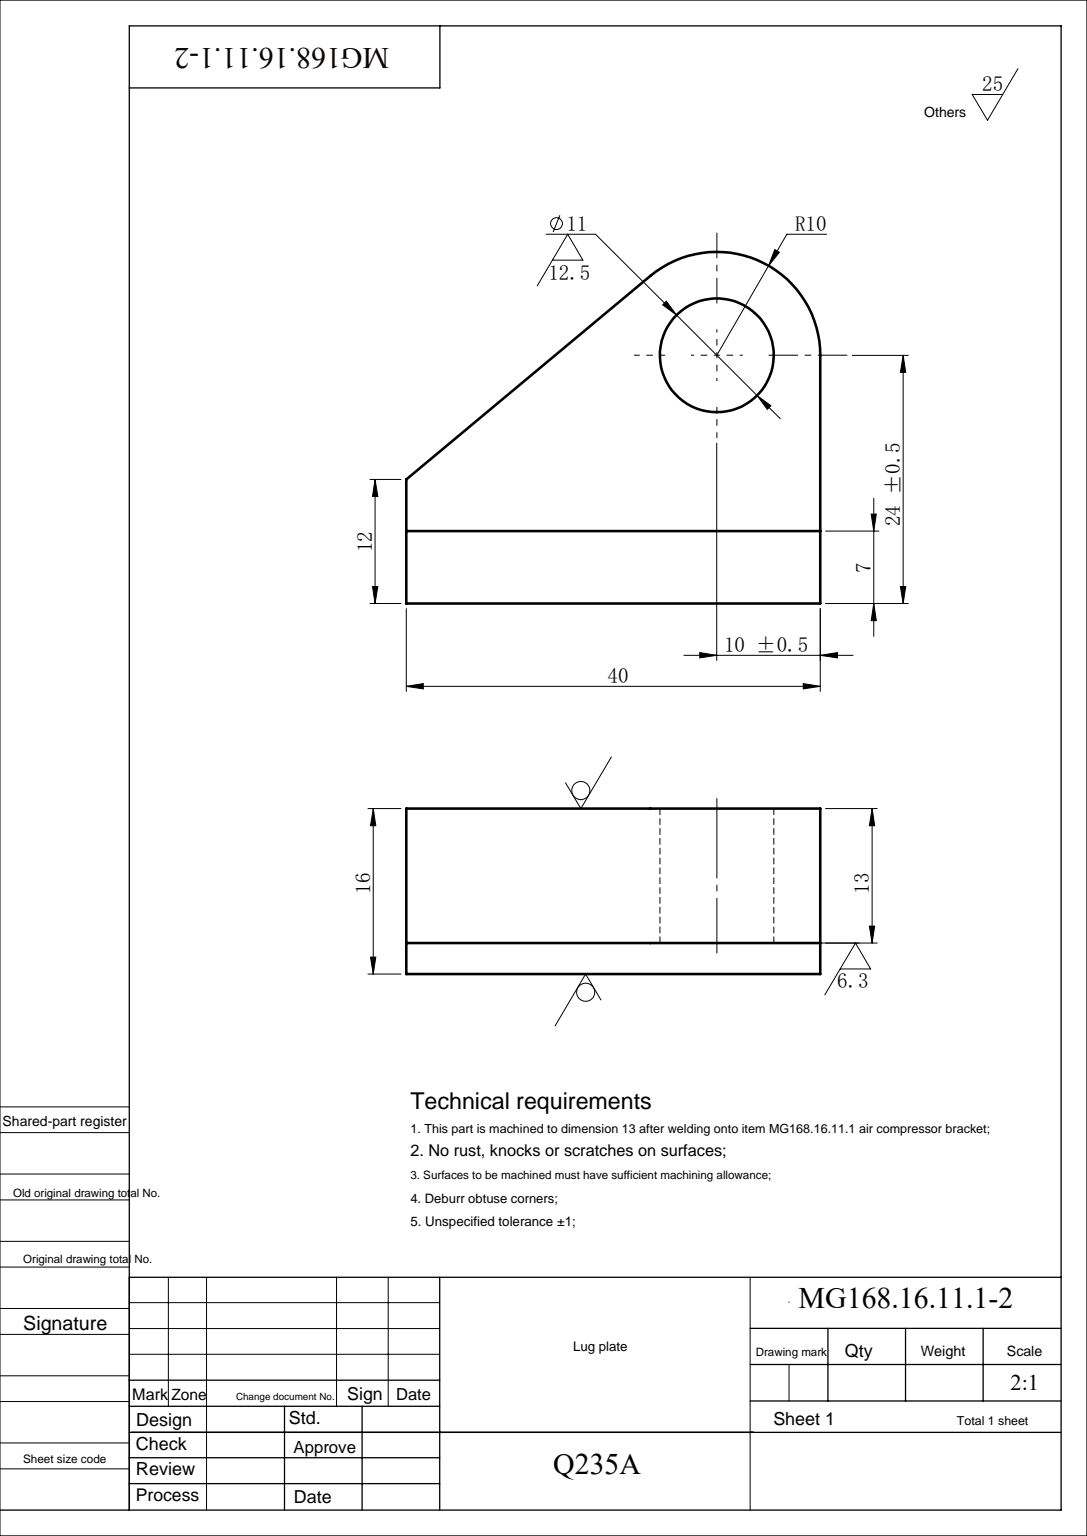
SolidWorks part; units mm, degrees
material "Q235A"
ref_plane "Front Plane" through (0, 0, 0) normal (0, 0, 1) x (1, 0, 0)
ref_plane "Top Plane" through (0, 0, 0) normal (0, 1, 0) x (1, 0, 0)
ref_plane "Right Plane" through (0, 0, 0) normal (1, 0, 0) x (0, 0, -1)
sketch "Sketch1" plane through (0, 0, 0) normal (0, 1, 0) x (1, 0, 0)
  line L0 (40, 12) -> (16.4051, 31.6795)
  line L1 (0, 0) -> (40, 0)
  line L2 (0, 0) -> (0, 24)
  line L4 (40, 0) -> (40, 12)
  arc A0 (0, 24) -> (16.4051, 31.6795) centre (10, 24) cw
  circle A1 centre (10, 24) radius 5.5
  dimension "D1" = 40
  dimension "D4" = 10
  dimension "D5" = 11
  dimension "D2" = 12
  dimension "D3" = 24
extrude "Boss-Extrude1" add sketch "Sketch1" along normal mid plane 13
sketch "Sketch2" plane through (0, -6.5, 0) normal (0, 1, 0) x (1, 0, 0)
  line L0 (40, 0) -> (40, 12) construction
  line L1 (0, 0) -> (40, 0)
  line L2 (0, 0) -> (0, 7)
  line L3 (0, 7) -> (40, 7)
  line L4 (40, 0) -> (40, 7)
  dimension "D1" = 7
extrude "Boss-Extrude2" add sketch "Sketch2" against normal blind 3
